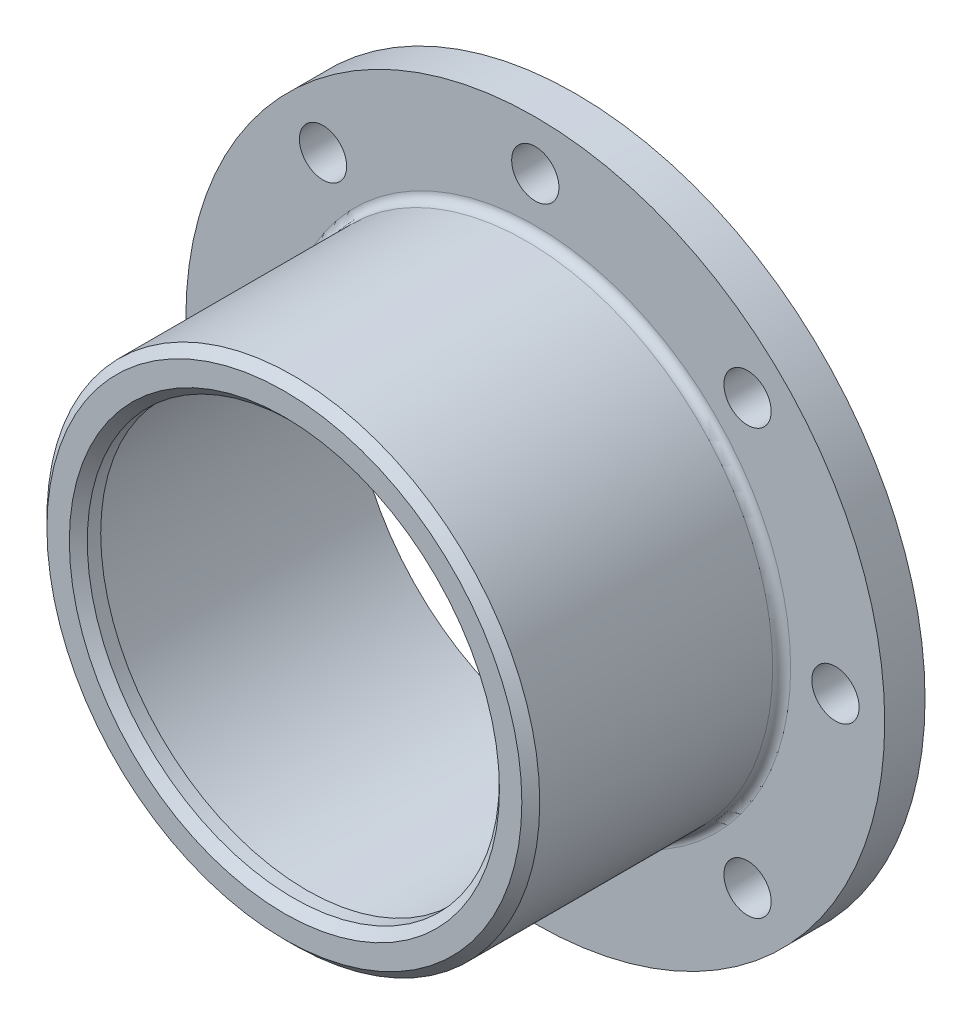
SolidWorks part; units mm, degrees
ref_plane "Front Plane" through (0, 0, 0) normal (0, 0, 1) x (1, 0, 0)
ref_plane "Top Plane" through (0, 0, 0) normal (0, 1, 0) x (1, 0, 0)
ref_plane "Right Plane" through (0, 0, 0) normal (1, 0, 0) x (0, 0, -1)
other "Configuration Table"
sketch "Sketch1" plane through (0, 0, 0) normal (0, 0, 1) x (1, 0, 0)
  circle A0 centre (0, 0) radius 78
  dimension "D1" = 156
extrude "Boss-Extrude1" add sketch "Sketch1" along normal blind 9
sketch "Sketch2" plane through (0, 0, 9) normal (0, 0, 1) x (1, 0, 0)
  circle A0 centre (0, 0) radius 55
  dimension "D1" = 110
extrude "Boss-Extrude2" add sketch "Sketch2" along normal blind 56
sketch "Sketch3" plane through (0, 0, 0) normal (0, 0, -1) x (-1, 0, 0)
  circle A0 centre (0, 0) radius 50
  dimension "D1" = 100
extrude "Cut-Extrude2" cut sketch "Sketch3" against normal blind 60
sketch "Sketch4" plane through (0, 0, 65) normal (0, 0, 1) x (1, 0, 0)
  circle A0 centre (0, 0) radius 46
  dimension "D1" = 92
extrude "Cut-Extrude3" cut sketch "Sketch4" against normal through all contours A0
sketch "Sketch5" plane through (0, 0, 0) normal (0, 0, -1) x (-1, 0, 0)
  circle A0 centre (0, 0) radius 67 construction
  circle A1 centre (0, 67) radius 5.275
  dimension "D1" = 134
  dimension "D2" = 10.55
extrude "Cut-Extrude4" cut sketch "Sketch5" against normal through all
pattern_circular "CirPattern1" count 8 over 360 about axis through (0, 0, 0) along (0, 0, 1) of "Cut-Extrude4"
chamfer "Chamfer1" distance 2 angle 45 2 edges at (55, 0, 65) (46, 0, 65)
fillet "Fillet1" radius 2 1 edges at (55, 0, 9)
